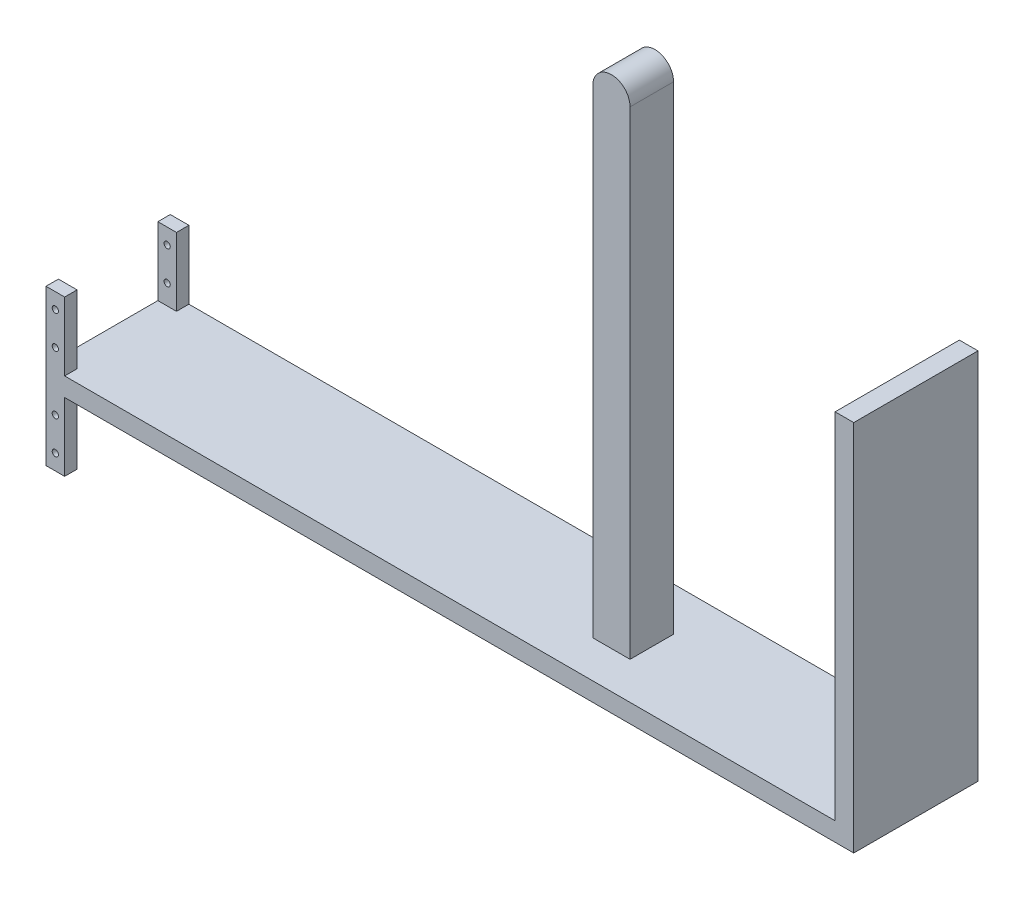
from build123d import *

# Parameters (mm, degrees)
BOSS_EXTRUDE1_DEPTH = 200
SKETCH4_W           = 20
SKETCH4_H           = 250
BOSS_EXTRUDE2_DEPTH = 30
SKETCH5_R           = 5
CUT_EXTRUDE1_DEPTH  = 230
BOSS_EXTRUDE5_START = -60
BOSS_EXTRUDE5_DEPTH = 70


with BuildPart() as part:
    # Sketch2 → Boss-Extrude1 (new body)
    with BuildSketch(Plane.XY):
        Polygon((-148.050188004, -835.198427503), (-178.050188004, -835.198427503), (-178.050188004, -1405.198427503), (-1448.050188004, -1405.198427503), (-1448.050188004, -1435.198427503), (-148.050188004, -1435.198427503), align=None)
    extrude(amount=-BOSS_EXTRUDE1_DEPTH)

    # Sketch4 → Boss-Extrude2 (add)
    with BuildSketch(Plane.ZY.offset(1448.050188004)):
        with Locations((-190, -1420.198427503)):
            Rectangle(SKETCH4_W, SKETCH4_H)
        with Locations((-10, -1420.198427503)):
            Rectangle(SKETCH4_W, SKETCH4_H)
    extrude(amount=-BOSS_EXTRUDE2_DEPTH)

    # Sketch5 → Cut-Extrude1 (cut)
    with BuildSketch(Plane(origin=(0, 0, -200), x_dir=(-1, 0, 0), z_dir=(0, 0, -1))):
        with Locations((1433.050188004, -1320.198427503)):
            Circle(SKETCH5_R)
        with Locations((1433.050188004, -1373.198427503)):
            Circle(SKETCH5_R)
        with Locations((1433.050188004, -1520.198427503)):
            Circle(SKETCH5_R)
        with Locations((1433.050188004, -1467.198427503)):
            Circle(SKETCH5_R)
    extrude(amount=-CUT_EXTRUDE1_DEPTH, mode=Mode.SUBTRACT)

    # Sketch9 → Boss-Extrude5 (add)
    with BuildSketch(Plane.XY.offset(BOSS_EXTRUDE5_START)):
        with BuildLine():
            Line((-568.050188004, -1405.198427503), (-628.050188004, -1405.198427503))
            Line((-628.050188004, -1405.198427503), (-628.050188004, -635.198427503))
            ThreePointArc((-628.050188004, -635.198427503), (-598.050188004, -605.198427503), (-568.050188004, -635.198427503))
            Line((-568.050188004, -635.198427503), (-568.050188004, -1405.198427503))
        make_face()
    extrude(amount=-BOSS_EXTRUDE5_DEPTH)


solid = part.part
